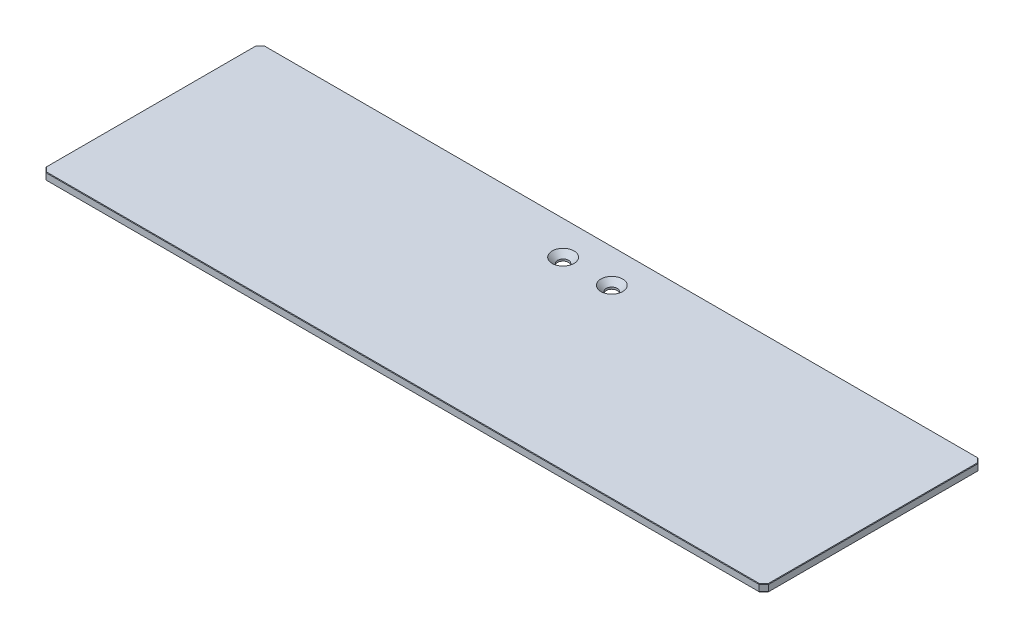
from build123d import *

# Parameters (mm, degrees)
SKETCH_1_W                  = 297
SKETCH_1_H                  = 90
EXTRUDE_1_DEPTH             = 3
HOLE_WIZARD_M4_1_AT_2_COUNT = 2
HOLE_WIZARD_M4_1_AT_2_PITCH = 20
CHAMFER_1_SIZE              = 2
CHAMFER_2_SIZE              = 0.2
CHAMFER_3_SIZE              = 0.2


with BuildPart() as part:
    # 草图1 → 凸台-拉伸1 (new body)
    with BuildSketch(Plane(origin=(0, 0, 0), x_dir=(1, 0, 0), z_dir=(0, 1, 0))):
        Rectangle(SKETCH_1_W, SKETCH_1_H)
    extrude(amount=EXTRUDE_1_DEPTH)

    # 草图2 → M4 六角凹锥坑螺钉的锥形沉头孔1 (revolve, cut)
    with BuildSketch(Plane(origin=(-10, 3, -31), x_dir=(0, 0, 1), z_dir=(1, 0, 0))):
        Polygon((0, 0), (0, 3), (2.25, 3), (2.25, 2.23), (4.48, 0), align=None)
    hole_wizard_m4_1 = revolve(axis=Axis((-10, 9.35, -31), (0, -1, 0)), mode=Mode.SUBTRACT)

    # M4 六角凹锥坑螺钉的锥形沉头孔1 at 2: M4 六角凹锥坑螺钉的锥形沉头孔1 ×2
    with Locations(*[(i * HOLE_WIZARD_M4_1_AT_2_PITCH, 0, 0) for i in range(1, HOLE_WIZARD_M4_1_AT_2_COUNT)]):
        add(hole_wizard_m4_1, mode=Mode.SUBTRACT)

    # 倒角1
    chamfer_1_edges = [part.edges().sort_by_distance(p)[0] for p in [
        (148.5, 1.5, 45),
        (-148.5, 1.5, 45),
        (-148.5, 1.5, -45),
        (148.5, 1.5, -45),
    ]]
    chamfer(chamfer_1_edges, length=CHAMFER_1_SIZE)

    # 倒角2
    chamfer_2_edges = [part.edges().sort_by_distance(p)[0] for p in [
        (0, 0, -45),
        (148.5, 0, 0),
        (0, 0, 45),
        (-148.5, 0, 0),
        (-147.5, 0, -44),
        (-147.5, 0, 44),
        (147.5, 0, 44),
        (147.5, 0, -44),
    ]]
    chamfer(chamfer_2_edges, length=CHAMFER_2_SIZE)

    # 倒角3
    chamfer_3_edges = [part.edges().sort_by_distance(p)[0] for p in [
        (0, 3, -45),
        (148.5, 3, 0),
        (-148.5, 3, 0),
        (0, 3, 45),
        (-147.5, 3, -44),
        (-147.5, 3, 44),
        (147.5, 3, 44),
        (147.5, 3, -44),
    ]]
    chamfer(chamfer_3_edges, length=CHAMFER_3_SIZE)


solid = part.part
